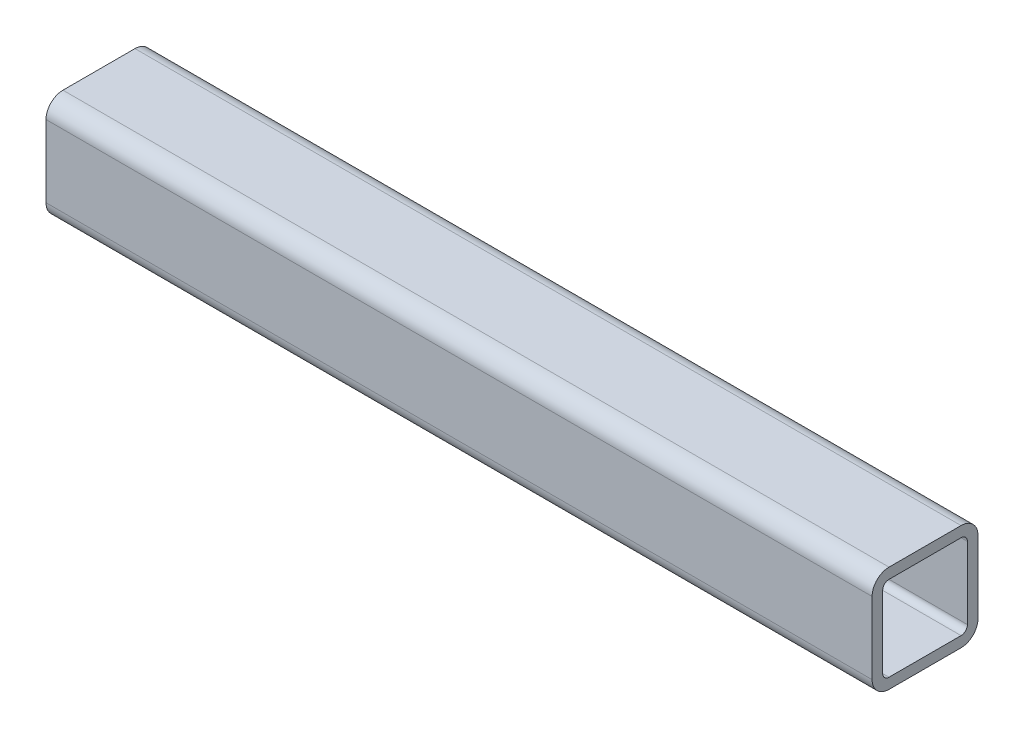
from build123d import *

# Parameters (mm, degrees)
COLD_FORMED_SQUARE_HOLLOW_SECTION_GB_T_6_DEPTH = 390


with BuildPart() as part:
    # Sketch1 → Cold-formed square hollow section GB/T 6728-2002 50 X 50 X 4(1) (new body)
    with BuildSketch(Plane.YZ.offset(-88.434077868)):
        with BuildLine():
            Line((-17, -25), (17, -25))
            ThreePointArc((17, -25), (22.656854249, -22.656854249), (25, -17))
            Line((25, -17), (25, 17))
            ThreePointArc((25, 17), (22.656854249, 22.656854249), (17, 25))
            Line((17, 25), (-17, 25))
            ThreePointArc((-17, 25), (-22.656854249, 22.656854249), (-25, 17))
            Line((-25, 17), (-25, -17))
            ThreePointArc((-25, -17), (-22.656854249, -22.656854249), (-17, -25))
        make_face()
        with BuildLine():
            Line((-17, -20), (17, -20))
            ThreePointArc((17, -20), (19.121320344, -19.121320344), (20, -17))
            Line((20, -17), (20, 17))
            ThreePointArc((20, 17), (19.121320344, 19.121320344), (17, 20))
            Line((17, 20), (-17, 20))
            ThreePointArc((-17, 20), (-19.121320344, 19.121320344), (-20, 17))
            Line((-20, 17), (-20, -17))
            ThreePointArc((-20, -17), (-19.121320344, -19.121320344), (-17, -20))
        make_face(mode=Mode.SUBTRACT)
    extrude(amount=COLD_FORMED_SQUARE_HOLLOW_SECTION_GB_T_6_DEPTH)


solid = part.part
